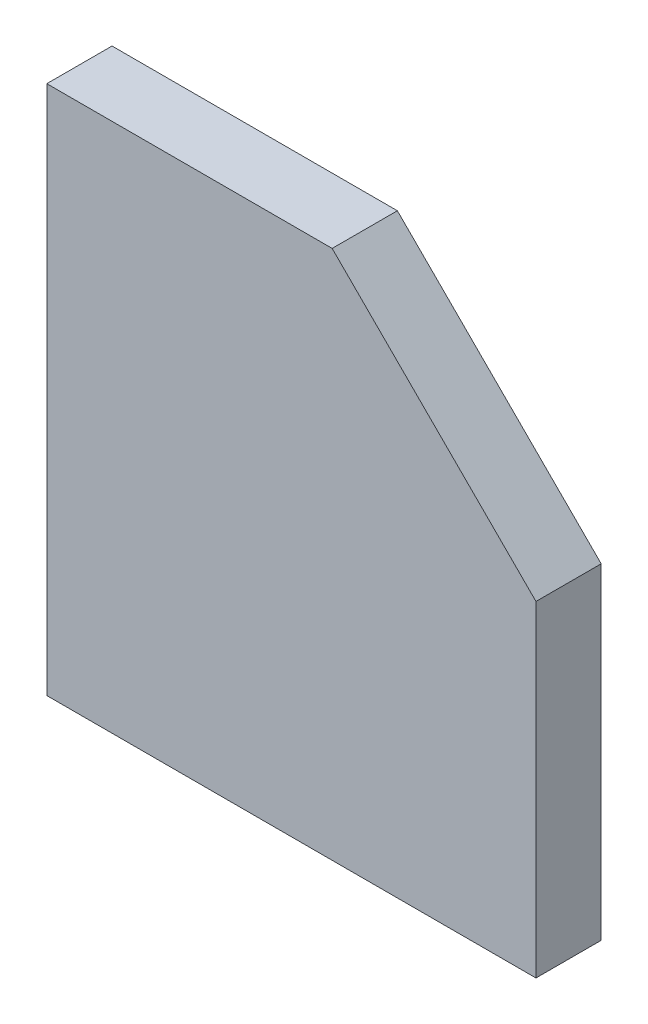
from build123d import *

# Parameters (mm, degrees)
SKETCH1_W           = 120
SKETCH1_H           = 130
BOSS_EXTRUDE1_DEPTH = 8
CHAMFER1_SIZE       = 50


with BuildPart() as part:
    # Sketch1 → Boss-Extrude1 (new, symmetric)
    with BuildSketch(Plane.XY):
        with Locations((60, 65)):
            Rectangle(SKETCH1_W, SKETCH1_H)
    extrude(amount=BOSS_EXTRUDE1_DEPTH, both=True)

    # Chamfer1
    chamfer1_edges = [part.edges().sort_by_distance(p)[0] for p in [
        (120, 130, 0),
    ]]
    chamfer(chamfer1_edges, length=CHAMFER1_SIZE)


solid = part.part
